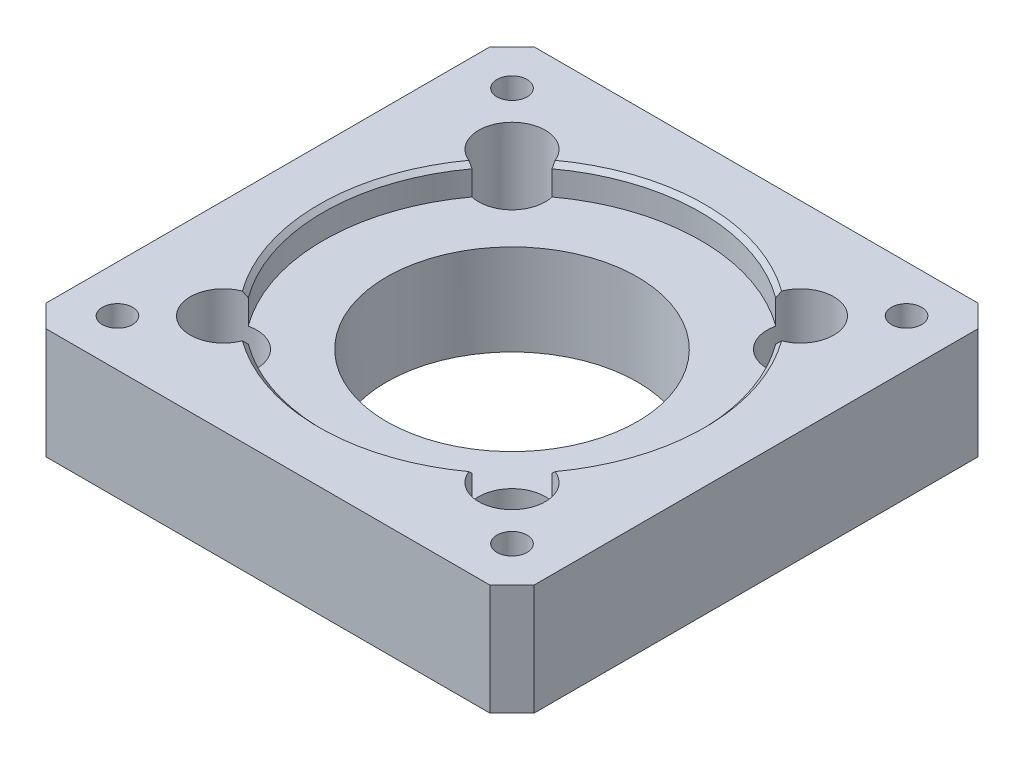
SolidWorks part; units mm, degrees
material "6061Al"
ref_plane "前视基准面" through (0, 0, 0) normal (0, 0, 1) x (1, 0, 0)
ref_plane "上视基准面" through (0, 0, 0) normal (0, 1, 0) x (1, 0, 0)
ref_plane "右视基准面" through (0, 0, 0) normal (1, 0, 0) x (0, 0, -1)
sketch "草图1" plane through (0, 0, 0) normal (0, 1, 0) x (1, 0, 0)
  line L1 (-55, -55) -> (55, -55)
  line L2 (-55, -55) -> (-55, 55)
  line L3 (-55, 55) -> (55, 55)
  line L4 (55, -55) -> (55, 55)
  line L5 (-55, -55) -> (55, 55) construction
  line L6 (-55, 55) -> (55, -55) construction
  point P0 (0, 0)
  dimension "D1" = 110
extrude "凸台-拉伸1" add sketch "草图1" along normal blind 25
sketch "草图3" plane through (0, 0, 0) normal (0, -1, 0) x (1, 0, 0)
  circle A0 centre (0, 0) radius 31.25
  circle A1 centre (0, 0) radius 28.25
  dimension "D1" = 62.5
  dimension "D2" = 3
extrude "凸台-拉伸2" add sketch "草图3" along normal blind 2
sketch "草图4" plane through (0, 0, 0) normal (0, -1, 0) x (1, 0, 0)
  circle A1 centre (0, 0) radius 28.25
  circle A2 centre (0, 0) radius 28.25
  dimension "D1" = 0
extrude "切除-拉伸1" cut sketch "草图4" against normal through all
sketch "草图5" plane through (0, 25, 0) normal (0, 1, 0) x (1, 0, 0)
  circle A0 centre (0, 0) radius 42.5
  dimension "D1" = 85
extrude "切除-拉伸2" cut sketch "草图5" against normal blind 6.5
hole_wizard "M8 螺纹孔1" positions "草图6" profile "草图7" tap size "M8" standard "ISO"
sketch "草图6" plane through (0, 25, 0) normal (0, 1, 0) x (1, 0, 0)
  line L1 (-44.45, -44.45) -> (44.45, -44.45)
  line L2 (-44.45, -44.45) -> (-44.45, 44.45)
  line L3 (-44.45, 44.45) -> (44.45, 44.45)
  line L4 (44.45, -44.45) -> (44.45, 44.45)
  line L5 (-44.45, -44.45) -> (44.45, 44.45) construction
  line L6 (-44.45, 44.45) -> (44.45, -44.45) construction
  point P0 (-44.45, 44.45)
  point P3 (0, 0)
  point P4 (44.45, 44.45)
  point P7 (-44.45, -44.45)
  point P31 (44.45, -44.45)
  dimension "D1" = 88.9
sketch "草图7" plane through (-44.45, 25, -44.45) normal (1, 0, 0) x (0, 0, 1)
  line L0 (0, 0) -> (0, 21.7929)
  line L1 (0, 21.7929) -> (3.4, 19.75)
  line L2 (3.4, 19.75) -> (3.4, 0)
  line L5 (3.4, 0) -> (0, 0)
  line L10 (0, 21.7929) -> (-3.4, 19.75) construction
  line L11 (0, -6.35) -> (0, 107.95) construction
  dimension "螺纹孔钻头直径" = 6.8
  dimension "螺纹孔钻头深度" = 19.75
  dimension "导头角度" = 118
cosmetic thread "孔螺蚊线1" parameters "D1"=16, "D2"=8
cosmetic thread "孔螺蚊线2" parameters "D1"=16, "D2"=8
cosmetic thread "孔螺蚊线3" parameters "D1"=16, "D2"=8
cosmetic thread "孔螺蚊线4" parameters "D1"=16, "D2"=8
hole_wizard "M8 六角凹头螺钉的柱形沉头孔1" positions "草图8" profile "草图9" counterbore size "M8" standard "ISO" end condition through all
sketch "草图8" plane through (0, 25, 0) normal (0, 1, 0) x (1, 0, 0)
  line L1 (-32.5, -32.5) -> (32.5, -32.5)
  line L2 (-32.5, -32.5) -> (-32.5, 32.5)
  line L3 (-32.5, 32.5) -> (32.5, 32.5)
  line L4 (32.5, -32.5) -> (32.5, 32.5)
  line L5 (-32.5, -32.5) -> (32.5, 32.5) construction
  line L6 (-32.5, 32.5) -> (32.5, -32.5) construction
  point P0 (-32.5, 32.5)
  point P3 (0, 0)
  point P4 (32.5, 32.5)
  point P7 (-32.5, -32.5)
  point P9 (32.5, -32.5)
  dimension "D1" = 65
sketch "草图9" plane through (-32.5, 25, -32.5) normal (1, 0, 0) x (0, 0, 1)
  line L0 (0, 0) -> (0, 27)
  line L1 (0, 27) -> (4.5, 27)
  line L3 (4.5, 27) -> (4.5, 18)
  line L4 (4.5, 18) -> (7.5, 18)
  line L5 (7.5, 18) -> (7.5, 0)
  line L7 (7.5, 0) -> (0, 0)
  line L11 (0, -6.35) -> (0, 107.95) construction
  dimension "通孔孔直径" = 9
  dimension "通孔孔深度" = 27
  dimension "柱形沉头孔直径" = 15
  dimension "柱形沉头孔深度" = 18
chamfer "倒角1" distance 5 angle 45 4 edges at (-55, 12.5, -55) (55, 12.5, -55) (55, 12.5, 55) (-55, 12.5, 55)
chamfer "倒角2" distance 1 angle 45 4 edges at (-42.5, 25, 0) (0, 25, -42.5) (42.5, 25, 0) (0, 25, 42.5)
chamfer "倒角3" distance 0.5 angle 45 1 edges at (0, -2, -31.25)
